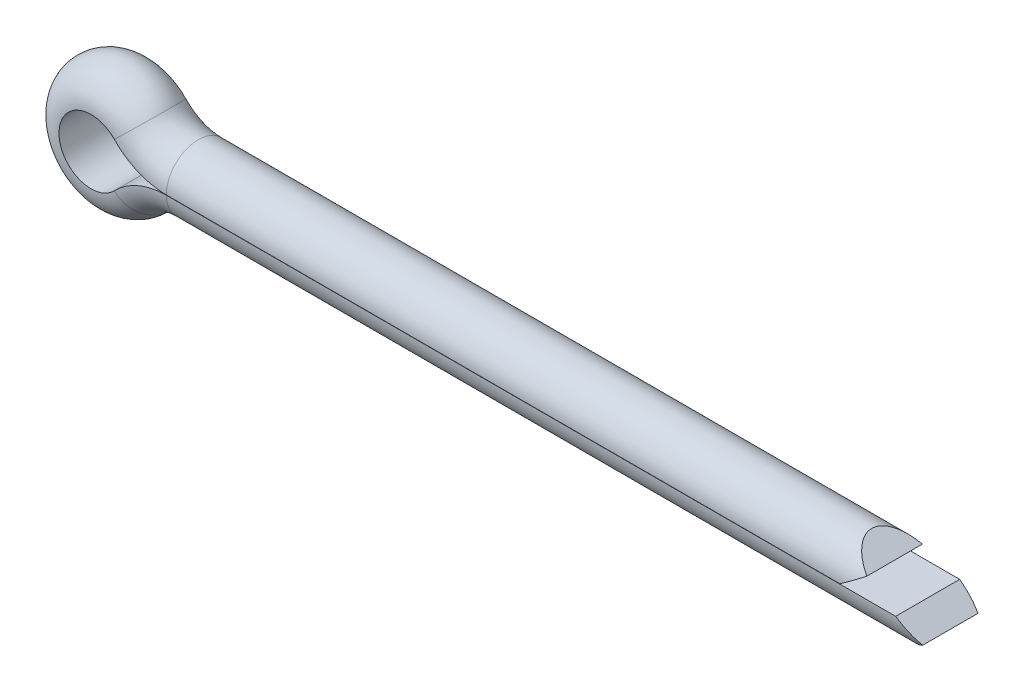
SolidWorks part; units mm, degrees
material "Q235"
ref_plane "Front Plane" through (0, 0, 0) normal (0, 0, 1) x (1, 0, 0)
ref_plane "Top Plane" through (0, 0, 0) normal (0, 1, 0) x (1, 0, 0)
ref_plane "Right Plane" through (0, 0, 0) normal (1, 0, 0) x (0, 0, -1)
sketch "Dimension sketch" plane through (0, 0, 0) normal (0, 0, 1) x (1, 0, 0)
  line L0 (55.4, 2.3) -> (5.4, 2.3)
  line L1 (5.4, -2.3) -> (59.4, -2.3)
  line L2 (5.4, 0) -> (27.3859, 0) construction
  line L3 (5.4, 0) -> (5.4, -0.0723) construction
  line L4 (-4.6, 0) -> (-4.6, 18.8979) construction
  arc A0 (5.4, 2.3) -> (3.3168, 3.1873) centre (5.4, 5.1891) cw
  arc A1 (3.3168, 3.1873) -> (3.3168, -3.1873) centre (0, 0) ccw
  arc A2 (3.3168, -3.1873) -> (5.4, -2.3) centre (5.4, -5.1891) cw
  dimension "c" = 9.2
  dimension "d1" = 4.6
  dimension "b" = 10
  dimension "l" = 50
  dimension "a" = 4
ref_plane "Plane1" through (55.4, 2.3, 0) normal (-1, 0, 0) x (0, 0, 1)
sketch "Sketch2" plane through (55.4, 2.3, 0) normal (-1, 0, 0) x (0, 0, 1)
  line L0 (0, -6.9) -> (0, 2.3) construction
  line L1 (-2.3, -2.29) -> (2.3, -2.29)
  arc A0 (2.3, -2.29) -> (-2.3, -2.29) centre (0, -2.3) ccw
  dimension "d" = 4.6
  dimension "D1" = 0.01
sweep "Sweep2" add profiles "Sketch2" path "Dimension sketch"
sketch "Sketch3" plane through (0, 0, 0) normal (0, 0, 1) x (1, 0, 0)
  line L0 (5.4, 0) -> (5.4, 16.2682) construction
  line L1 (5.4, 0) -> (37.4999, 0) construction
  line L2 (59.4, -2.3) -> (59.4, -0.01) construction
  line L3 (55.4, 1.145) -> (53.7611, 2.3)
  line L4 (55.4, 2.3) -> (5.4, 2.3) construction
  line L5 (5.4, -2.3) -> (59.4, -2.3) construction
  line L6 (55.4, 1.145) -> (53.7541, 0)
  line L7 (59.4, -1.155) -> (57.7611, 0)
  line L9 (59.4, -1.155) -> (57.7541, -2.3)
  line L10 (57.7611, 0) -> (53.7541, 0)
  line L11 (53.7611, 2.3) -> (59.41, 2.3)
  line L12 (59.41, 2.3) -> (59.41, -2.3)
  line L13 (59.41, -2.3) -> (57.7541, -2.3)
  line L14 (55.4, 2.3) -> (55.4, 0.01) construction
  dimension "D1" = 0.01
  dimension "D3" = 70
  dimension "D4" = 70
extrude "Cut-Extrude1" cut sketch "Sketch3" against normal through all and the other way through all
